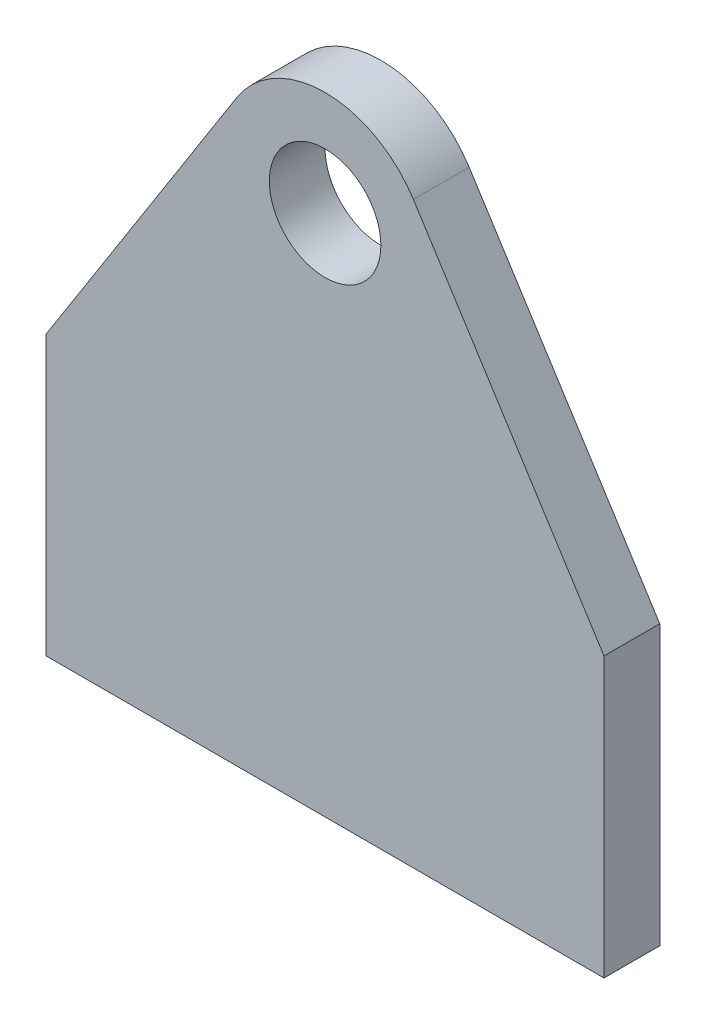
from build123d import *

# Parameters (mm, degrees)
SKETCH1_R           = 8
BOSS_EXTRUDE1_DEPTH = 8


with BuildPart() as part:
    # Sketch1 → Boss-Extrude1 (new body)
    with BuildSketch(Plane.XY):
        with BuildLine():
            Line((0, 0), (0, 40))
            Line((0, 40), (27.338105329, 83.042165339))
            ThreePointArc((27.338105329, 83.042165339), (40, 90), (52.661894671, 83.042165339))
            Line((52.661894671, 83.042165339), (80, 40))
            Line((80, 40), (80, 0))
            Line((80, 0), (0, 0))
        make_face()
        with Locations((40, 75)):
            Circle(SKETCH1_R, mode=Mode.SUBTRACT)
    extrude(amount=BOSS_EXTRUDE1_DEPTH)


solid = part.part
